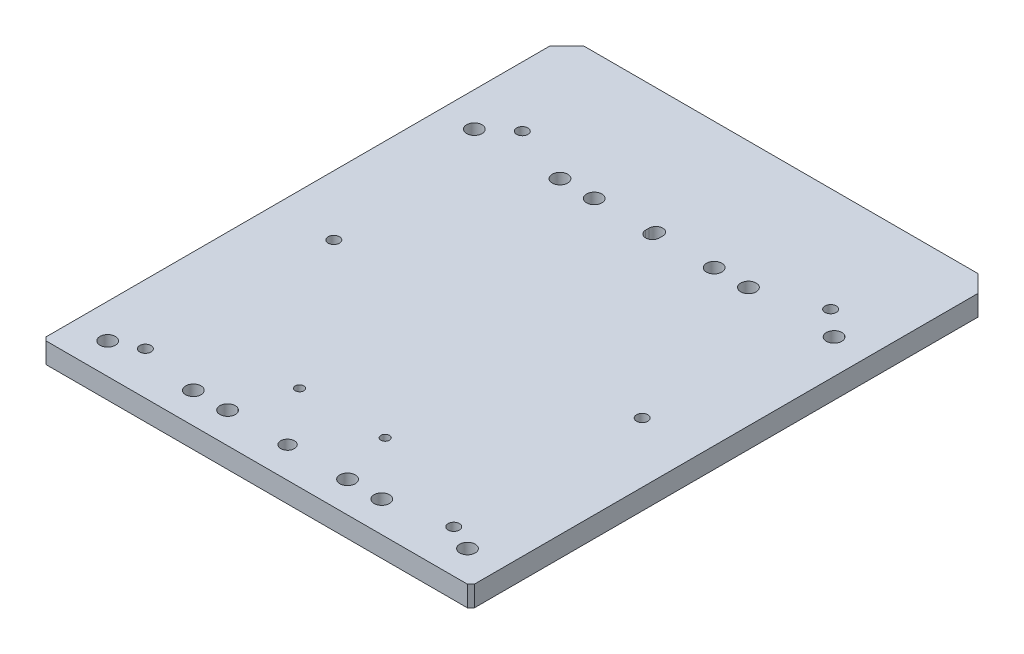
SolidWorks part; units mm, degrees
material "A6061"
ref_plane "前基準面" through (0, 0, 0) normal (0, 0, 1) x (1, 0, 0)
ref_plane "上基準面" through (0, 0, 0) normal (0, 1, 0) x (1, 0, 0)
ref_plane "右基準面" through (0, 0, 0) normal (1, 0, 0) x (0, 0, -1)
sketch "草图1" plane through (0, 0, 0) normal (0, 1, 0) x (1, 0, 0)
  line L1 (-125, -153) -> (125, -153)
  line L2 (-125, -153) -> (-125, 153)
  line L3 (-125, 153) -> (125, 153)
  line L4 (125, -153) -> (125, 153)
  line L5 (-125, -153) -> (125, 153) construction
  line L6 (-125, 153) -> (125, -153) construction
  point P0 (0, 0)
  dimension "D1" = 250
  dimension "D2" = 306
extrude "凸台-拉伸1" add sketch "草图1" along normal mid plane 12
chamfer "倒角1" distance 2 angle 45 2 edges at (125, 0, 153) (-125, 0, 153)
hole_wizard "M6 螺纹孔1" positions "草图2" profile "草图3" tap size "M6" standard "GB"
sketch "草图2" plane through (0, 0, -153) normal (0, 0, -1) x (-1, 0, 0)
  line L0 (0, 43.8121) -> (0, 0) construction
  point P0 (-105, 0)
  point P2 (0, 0)
  point P9 (105, 0)
  dimension "D1" = 210
sketch "草图3" plane through (105, 0, -153) normal (1, 0, 0) x (0, 1, 0)
  line L0 (0, 0) -> (0, 16.5022)
  line L1 (0, 16.5022) -> (2.5, 15)
  line L2 (2.5, 15) -> (2.5, 0)
  line L5 (2.5, 0) -> (0, 0)
  line L10 (0, 16.5022) -> (-2.5, 15) construction
  line L11 (0, -6.35) -> (0, 107.95) construction
  dimension "螺纹孔钻头直径" = 5
  dimension "螺纹孔钻头深度" = 15
  dimension "导头角度" = 118
cosmetic thread "孔螺蚊线1" parameters "D1"=12, "D2"=6
cosmetic thread "孔螺蚊线2" parameters "D1"=12, "D2"=6
cosmetic thread "孔螺蚊线3" parameters "D1"=12, "D2"=6
hole_wizard "M8 间隙孔1" positions "草图4" profile "草图5" hole size "M8" standard "GB" end condition through all
sketch "草图4" plane through (0, 6, 0) normal (0, 1, 0) x (1, 0, 0)
  line L0 (0, -216.6074) -> (0, 0) construction
  line L1 (-123, -153) -> (123, -153) construction
  point P0 (-105, -135)
  point P2 (-55, -135)
  point P4 (-105, 79)
  point P6 (-55, 79)
  point P11 (55, 79)
  point P12 (105, 79)
  point P13 (55, -135)
  point P14 (105, -135)
  point P17 (-35, -135)
  point P20 (35, -135)
  point P21 (-35, 79)
  point P24 (35, 79)
  dimension "D1" = 50
  dimension "D2" = 110
  dimension "D3" = 18
  dimension "D4" = 214
  dimension "D5" = 70
sketch "草图5" plane through (-105, 6, 135) normal (1, 0, 0) x (0, 0, 1)
  line L0 (0, 0) -> (0, 12)
  line L1 (0, 12) -> (4.5, 12)
  line L2 (4.5, 12) -> (4.5, 0)
  line L5 (4.5, 0) -> (0, 0)
  line L11 (0, -6.35) -> (0, 107.95) construction
  dimension "通孔孔直径" = 9
  dimension "通孔孔深度" = 12
hole_wizard "打孔尺寸(%根据)内六角圆柱头螺钉的类型1" positions "草图6" profile "草图7" counterbore size "M6" standard "GB" end condition through all
sketch "草图6" plane through (0, -6, 0) normal (0, -1, 0) x (-1, 0, 0)
  line L0 (123, -153) -> (-123, -153) construction
  line L1 (0, 0) -> (0, -200.2729) construction
  point P0 (-90, -128)
  point P8 (-90, -18)
  point P9 (-90, 92)
  point P20 (90, 92)
  point P21 (90, -18)
  point P22 (90, -128)
  dimension "D1" = 3
  dimension "D2" = 110
  dimension "D3" = 25
  dimension "D4" = 180
sketch "草图7" plane through (90, -6, 128) normal (1, 0, 0) x (0, 0, -1)
  line L0 (0, 0) -> (0, 12)
  line L1 (0, 12) -> (3.3, 12)
  line L3 (3.3, 12) -> (3.3, 6.8)
  line L4 (3.3, 6.8) -> (5.5, 6.8)
  line L5 (5.5, 6.8) -> (5.5, 0)
  line L7 (5.5, 0) -> (0, 0)
  line L11 (0, -6.35) -> (0, 107.95) construction
  dimension "通孔孔直径" = 6.6
  dimension "通孔孔深度" = 12
  dimension "柱形沉头孔直径" = 11
  dimension "柱形沉头孔深度" = 6.8
sketch "草图8" plane through (0, 6, 0) normal (0, 1, 0) x (1, 0, 0)
  line L0 (0, 78) -> (0, 80) construction
  line L1 (-4, 78) -> (-4, 80)
  line L2 (4, 78) -> (4, 80)
  line L3 (55, -135) -> (-55, -135) construction
  line L5 (55, 79) -> (-55, 79) construction
  circle A0 centre (0, -135) radius 4
  arc A1 (-4, 78) -> (4, 78) centre (0, 78) ccw
  arc A2 (4, 80) -> (-4, 80) centre (0, 80) ccw
  point P4 (0, 79)
  dimension "D1" = 8
  dimension "D2" = 2
extrude "切除-拉伸1" cut sketch "草图8" against normal through all
hole_wizard "M6 螺纹孔2" positions "草图9" profile "草图10" tap size "M6" standard "GB" end condition through all
sketch "草图9" plane through (0, 6, 0) normal (0, 1, 0) x (1, 0, 0)
  line L0 (0, -191.258) -> (0, 0) construction
  line L2 (-123, -153) -> (123, -153) construction
  point P0 (25, -103)
  point P2 (-25, -103)
  dimension "D1" = 50
  dimension "D3" = 50
sketch "草图10" plane through (25, 6, 103) normal (1, 0, 0) x (0, 0, 1)
  line L0 (0, 0) -> (0, 12)
  line L1 (0, 12) -> (2.5, 12)
  line L2 (2.5, 12) -> (2.5, 0)
  line L5 (2.5, 0) -> (0, 0)
  line L11 (0, -6.35) -> (0, 107.95) construction
  dimension "通孔螺纹孔钻头直径" = 5
  dimension "通孔螺纹孔钻头深度" = 12
cosmetic thread "孔螺蚊线6" parameters "D2"=6
cosmetic thread "孔螺蚊线7" parameters "D2"=6
hole_wizard "M8 间隙孔2" positions "草图11" profile "草图12" hole size "M8" standard "GB"
sketch "草图11" plane through (0, 6, 0) normal (0, 1, 0) x (1, 0, 0)
  line L0 (0, 0) -> (0, -173.9198) construction
  line L2 (-123, -153) -> (123, -153) construction
  point P4 (75, -83.0002)
  point P7 (75, 6.9998)
  point P9 (0, -83.0002)
  point P11 (0, 6.9998)
  point P18 (-75, 6.9998)
  point P19 (-75, -83.0002)
  dimension "D1" = 150
  dimension "D2" = 90
  dimension "D3" = 69.9998
sketch "草图12" plane through (75, 6, 83.0002) normal (1, 0, 0) x (0, 0, 1)
  line L0 (0, 0) -> (0, 12)
  line L1 (0, 12) -> (4.5, 12)
  line L2 (4.5, 12) -> (4.5, 0)
  line L5 (4.5, 0) -> (0, 0)
  line L11 (0, -6.35) -> (0, 107.95) construction
  dimension "通孔孔直径" = 9
  dimension "通孔孔深度" = 12
chamfer "倒角2" distance 10 angle 45 2 edges at (-125, 0, -153) (125, 0, -153)
